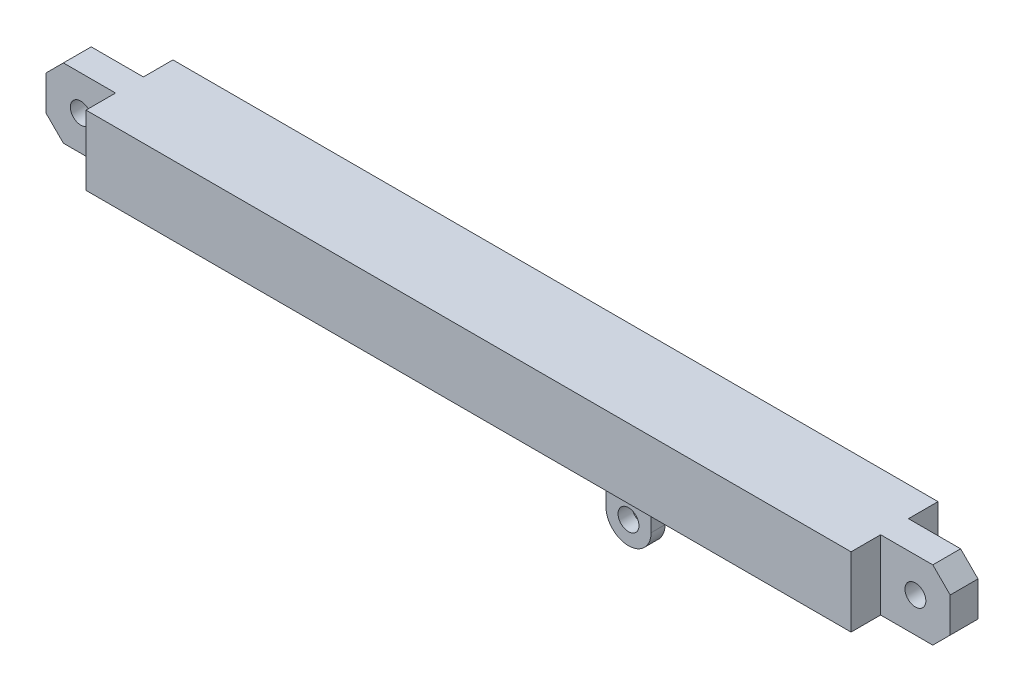
from build123d import *

# Parameters (mm, degrees)
SKETCH1_W           = 260
SKETCH1_H           = 20
BOSS_EXTRUDE1_DEPTH = 12.5
SKETCH2_R           = 3
CUT_EXTRUDE1_DEPTH  = 133.759180474
SKETCH3_W           = 20
SKETCH3_H           = 20
CUT_EXTRUDE2_DEPTH  = 8.5
CHAMFER1_SIZE       = 5
SKETCH4_R           = 3
BOSS_EXTRUDE2_DEPTH = 4
LPATTERN1_COUNT     = 2
LPATTERN1_PITCH     = 15


with BuildPart() as part:
    # Sketch1 → Boss-Extrude1 (new, symmetric)
    with BuildSketch(Plane.XY):
        Rectangle(SKETCH1_W, SKETCH1_H)
    extrude(amount=BOSS_EXTRUDE1_DEPTH, both=True)

    # Sketch2 → Cut-Extrude1 (cut, through all)
    with BuildSketch(Plane.XY.offset(12.5)):
        with Locations((-120, 0)):
            Circle(SKETCH2_R)
        with Locations((120, 0)):
            Circle(SKETCH2_R)
    extrude(amount=-CUT_EXTRUDE1_DEPTH, mode=Mode.SUBTRACT)

    # Sketch3 → Cut-Extrude2 (cut)
    with BuildSketch(Plane.XY.offset(12.5)):
        with Locations((-120, 0)):
            Rectangle(SKETCH3_W, SKETCH3_H)
        with Locations((120, 0)):
            Rectangle(SKETCH3_W, SKETCH3_H)
    cut_extrude2 = extrude(amount=-CUT_EXTRUDE2_DEPTH, mode=Mode.SUBTRACT)

    # Mirror2: Cut-Extrude2 across plane
    add(cut_extrude2.mirror(Plane.XY), mode=Mode.SUBTRACT)

    # Chamfer1
    chamfer1_edges = [part.edges().sort_by_distance(p)[0] for p in [
        (130, -10, 0),
        (-130, -10, 0),
        (-130, 10, 0),
        (130, 10, 0),
    ]]
    chamfer(chamfer1_edges, length=CHAMFER1_SIZE)

    # Sketch4 → Boss-Extrude2 (add)
    with BuildSketch(Plane(origin=(0, 0, -12.5), x_dir=(-1, 0, 0), z_dir=(0, 0, -1))):
        with BuildLine():
            Line((-46.5, -20), (-46.5, -10))
            Line((-46.5, -10), (-33.5, -10))
            Line((-33.5, -10), (-33.5, -20))
            ThreePointArc((-33.5, -20), (-40, -26.5), (-46.5, -20))
        make_face()
        with Locations((-40, -20)):
            Circle(SKETCH4_R, mode=Mode.SUBTRACT)
    boss_extrude2 = extrude(amount=-BOSS_EXTRUDE2_DEPTH)

    # LPattern1: Boss-Extrude2 ×2
    with Locations(*[(0, 0, i * LPATTERN1_PITCH) for i in range(1, LPATTERN1_COUNT)]):
        add(boss_extrude2)


solid = part.part
